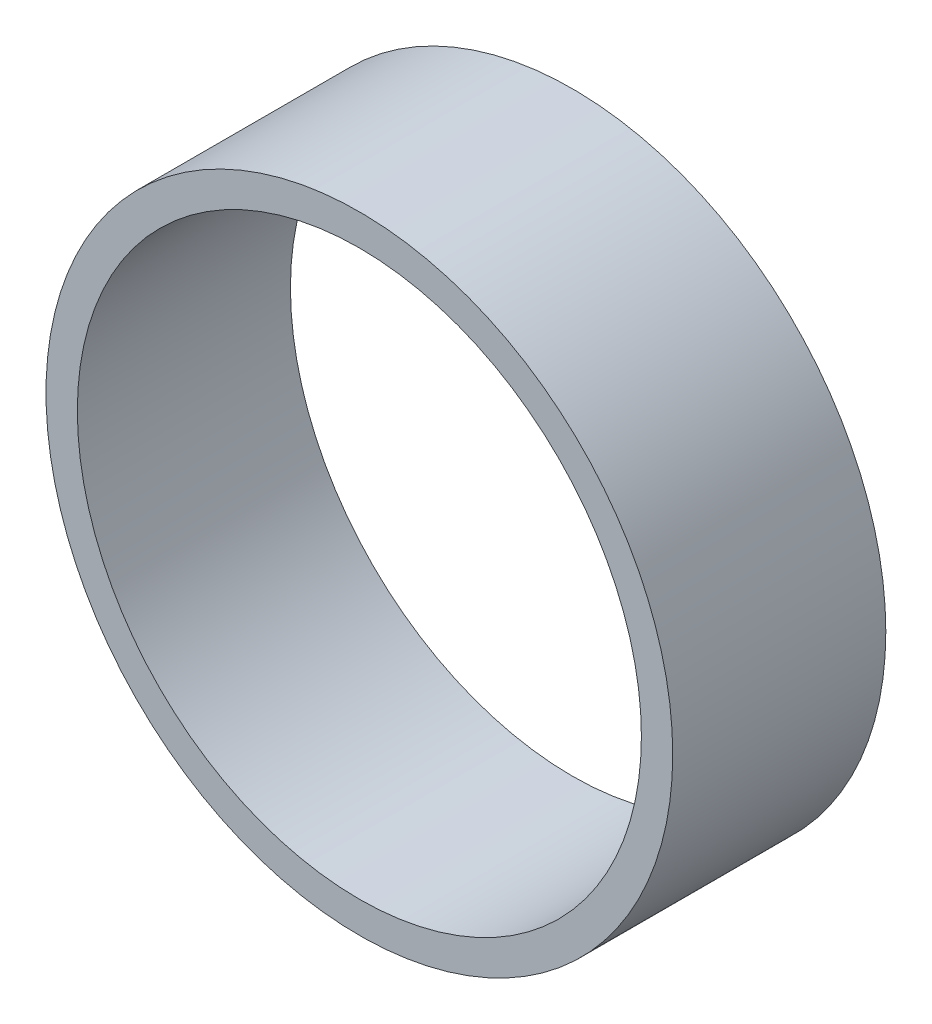
from build123d import *

# Parameters (mm, degrees)
SKETCH_1_R      = 50
SKETCH_1_R_2    = 45
EXTRUDE_1_DEPTH = 34


with BuildPart() as part:
    # 草图1 → 凸台-拉伸1 (new body)
    with BuildSketch(Plane.XY):
        Circle(SKETCH_1_R)
        Circle(SKETCH_1_R_2, mode=Mode.SUBTRACT)
    extrude(amount=EXTRUDE_1_DEPTH)


solid = part.part
